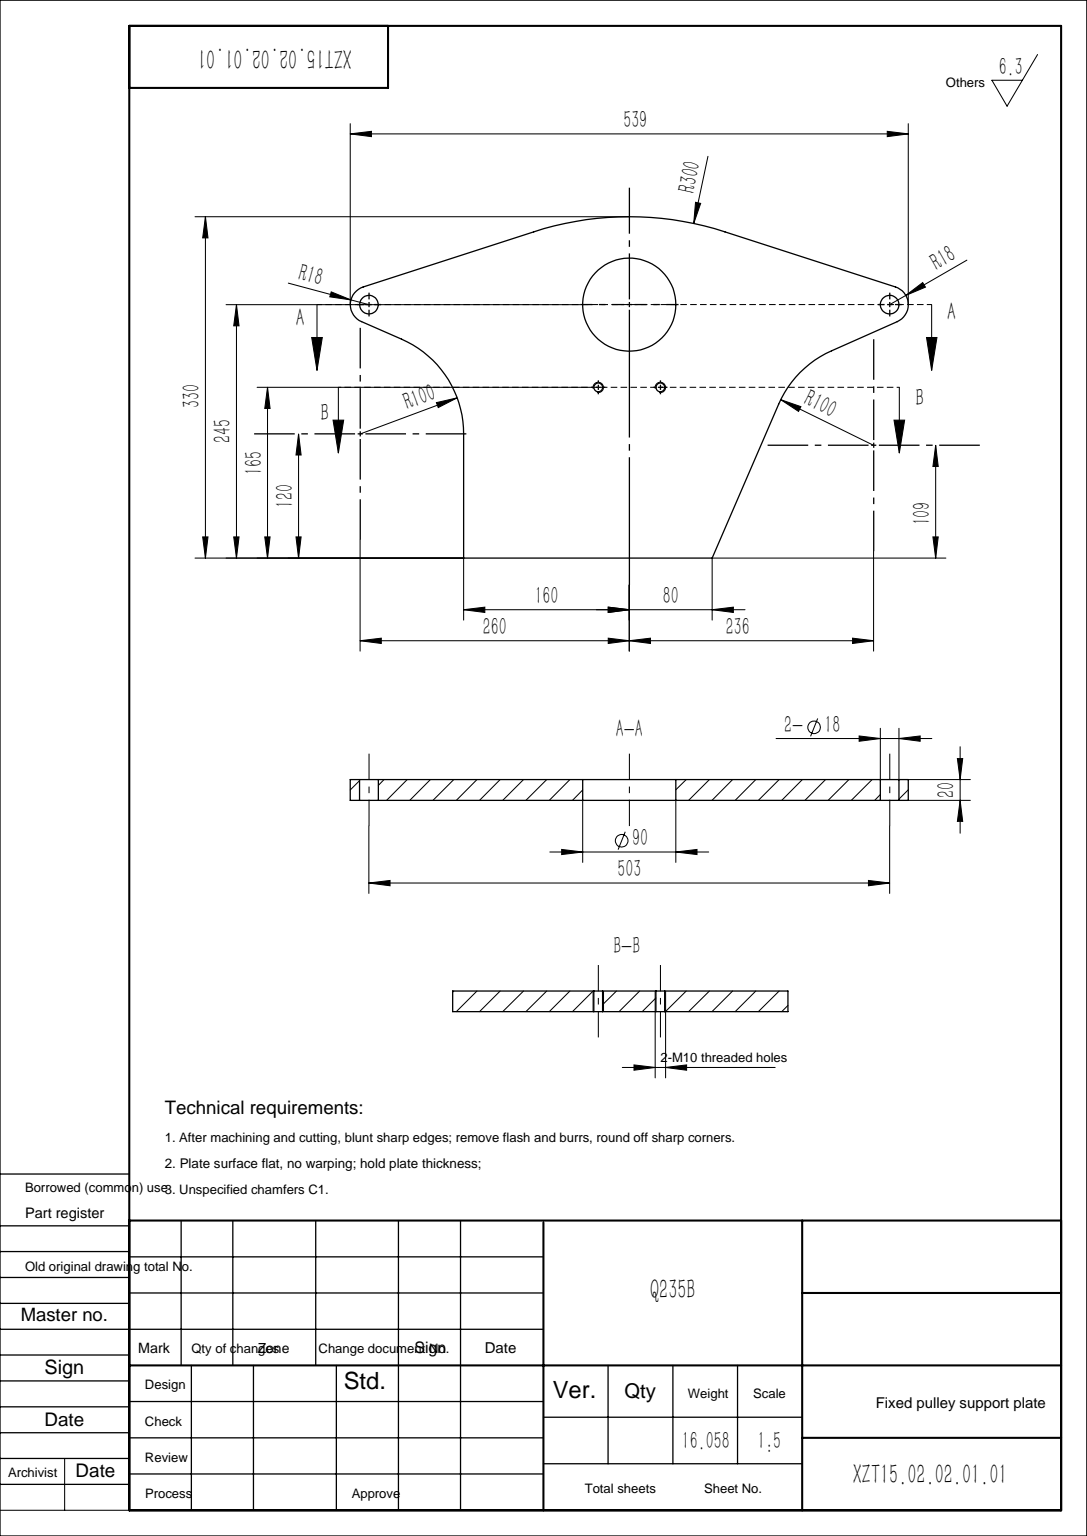
from build123d import *

# Parameters (mm, degrees)
SKETCH1_R           = 45
SKETCH1_R_2         = 9
BOSS_EXTRUDE1_DEPTH = 10
M10_TAPPED_HOLE1_D  = 8.5


with BuildPart() as part:
    # Sketch1 → Boss-Extrude1 (new, symmetric)
    with BuildSketch(Plane.XY):
        with BuildLine():
            Line((0, 0), (-160, 0))
            Line((-160, 0), (-160, 120))
            ThreePointArc((-160, 120), (-176.357134778, 174.807582481), (-220.077421949, 211.685264693))
            Line((-220.077421949, 211.685264693), (-258.686064049, 228.496652355))
            ThreePointArc((-258.686064049, 228.496652355), (-269.478553593, 245.878413735), (-257.04300386, 262.12527688))
            Line((-257.04300386, 262.12527688), (-92.383397673, 315.421281327))
            ThreePointArc((-92.383397673, 315.421281327), (0, 330), (92.383397673, 315.421281327))
            Line((92.383397673, 315.421281327), (257.04300386, 262.12527688))
            ThreePointArc((257.04300386, 262.12527688), (269.475222772, 245.944121974), (258.80651528, 228.549625097))
            Line((258.80651528, 228.549625097), (195.408248443, 200.390971685))
            ThreePointArc((195.408248443, 200.390971685), (164.925652867, 179.34512904), (144.195283074, 148.647117803))
            Line((144.195283074, 148.647117803), (80, 0))
            Line((80, 0), (0, 0))
        make_face()
        with Locations((0, 245)):
            Circle(SKETCH1_R, mode=Mode.SUBTRACT)
        with Locations((-251.5, 245)):
            Circle(SKETCH1_R_2, mode=Mode.SUBTRACT)
        with Locations((251.5, 245)):
            Circle(SKETCH1_R_2, mode=Mode.SUBTRACT)
    extrude(amount=BOSS_EXTRUDE1_DEPTH, both=True)

    # M10 Tapped Hole1 (through all)
    with Locations(Plane.XY.offset(10)):
        with Locations((-30, 165), (30, 165)):
            Hole(M10_TAPPED_HOLE1_D / 2)


solid = part.part
